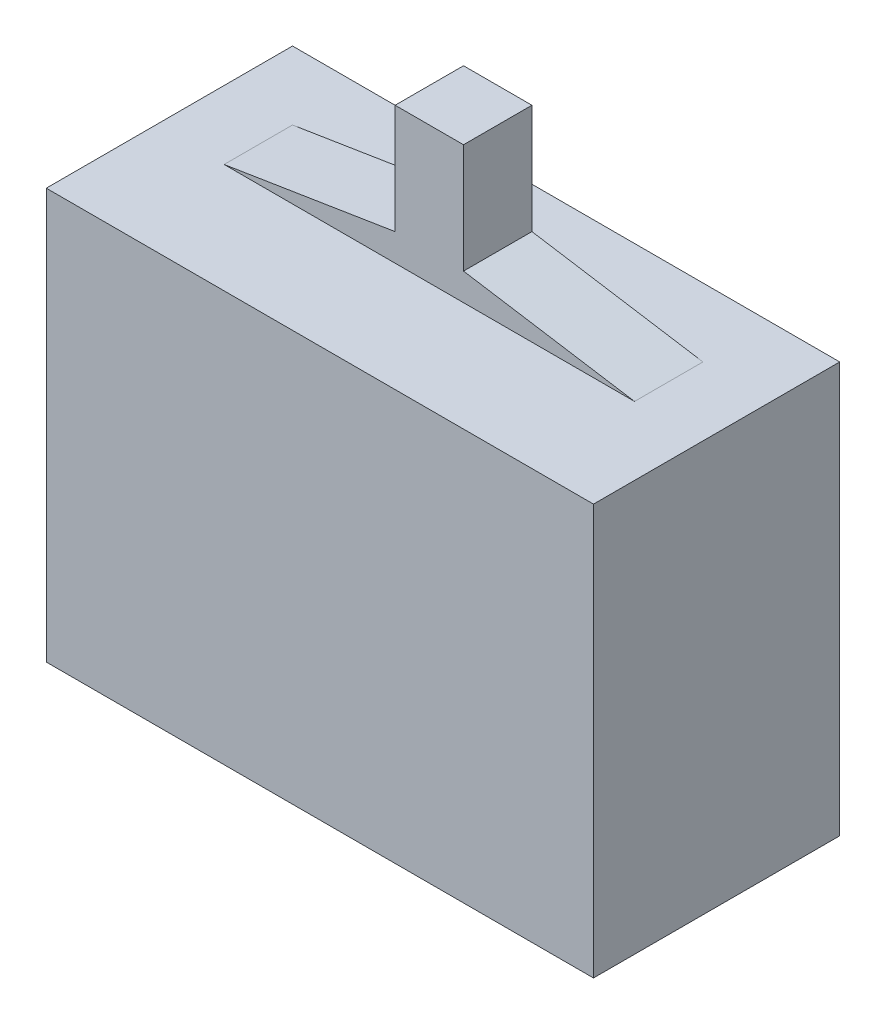
from build123d import *

# Parameters (mm, degrees)
SKETCH1_W           = 40
SKETCH1_H           = 30
BOSS_EXTRUDE1_DEPTH = 18
BOSS_EXTRUDE3_START = 5
BOSS_EXTRUDE3_DEPTH = 5


with BuildPart() as part:
    # Sketch1 → Boss-Extrude1 (new body)
    with BuildSketch(Plane.XY):
        with Locations((20, -15)):
            Rectangle(SKETCH1_W, SKETCH1_H)
    extrude(amount=BOSS_EXTRUDE1_DEPTH)

    # Sketch2 → Boss-Extrude3 (add)
    with BuildSketch(Plane.XY.offset(BOSS_EXTRUDE3_START)):
        Polygon((17.5, 10), (17.5, 2), (5, 0), (35, 0), (22.5, 2), (22.5, 10), align=None)
    extrude(amount=BOSS_EXTRUDE3_DEPTH)


solid = part.part
